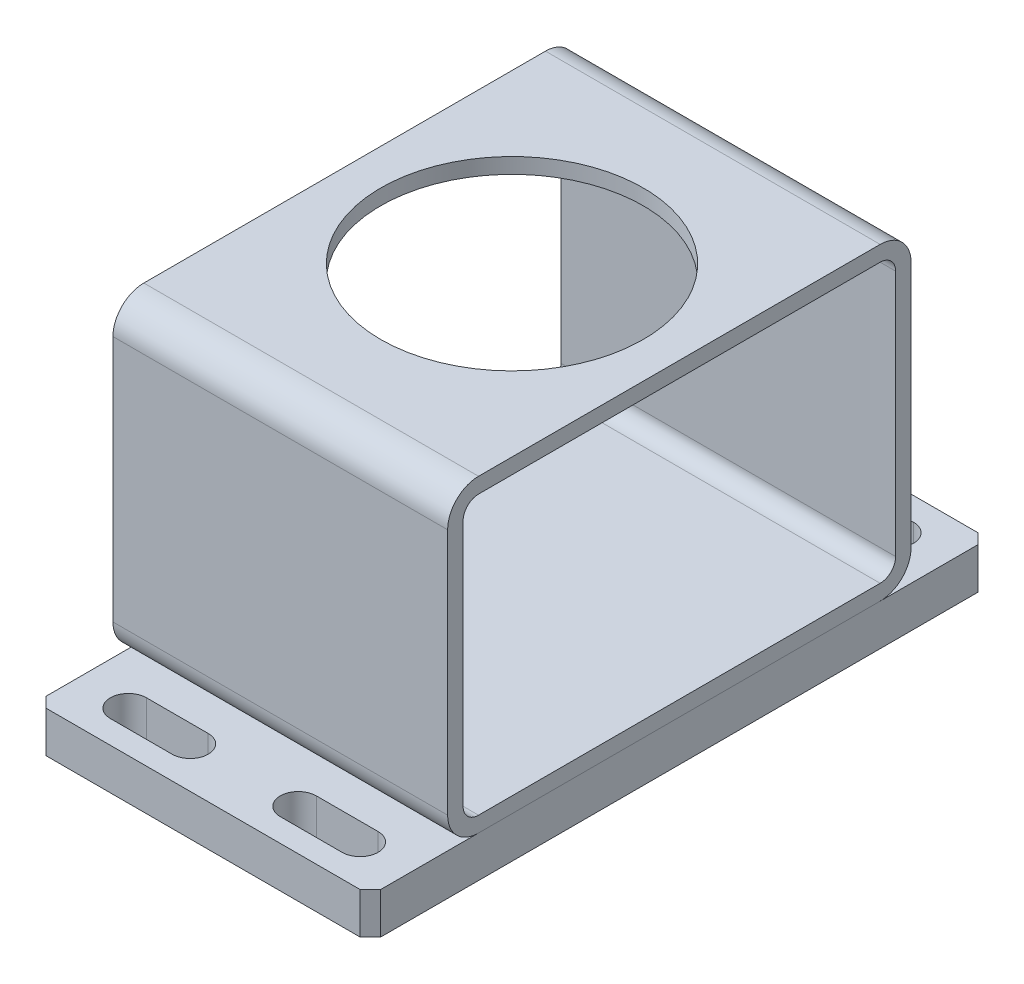
from build123d import *

# Parameters (mm, degrees)
GB_T6728_2002_90_X_60_X_3_1_DEPTH = 65
CUT_EXTRUDE_1_REACH               = 83.739
SKETCH_4_R                        = 25.5
SKETCH_7_W                        = 65
SKETCH_7_H                        = 120
EXTRUDE_1_DEPTH                   = 8
CUT_EXTRUDE_5_DEPTH               = 11
MIRROR_3_COPY_1_DEPTH             = 11
CHAMFER_1_SIZE                    = 2


with BuildPart() as part:
    # Sketch11 → 冷弯空心矩管gb∕t6728-2002 90 X 60 X 3(1) (new body)
    with BuildSketch(Plane.YZ.offset(-32.5)):
        with BuildLine():
            Line((-24, -45), (24, -45))
            ThreePointArc((24, -45), (28.242640687, -43.242640687), (30, -39))
            Line((30, -39), (30, 39))
            ThreePointArc((30, 39), (28.242640687, 43.242640687), (24, 45))
            Line((24, 45), (-24, 45))
            ThreePointArc((-24, 45), (-28.242640687, 43.242640687), (-30, 39))
            Line((-30, 39), (-30, -39))
            ThreePointArc((-30, -39), (-28.242640687, -43.242640687), (-24, -45))
        make_face()
        with BuildLine():
            Line((-24, -42), (24, -42))
            ThreePointArc((24, -42), (26.121320344, -41.121320344), (27, -39))
            Line((27, -39), (27, 39))
            ThreePointArc((27, 39), (26.121320344, 41.121320344), (24, 42))
            Line((24, 42), (-24, 42))
            ThreePointArc((-24, 42), (-26.121320344, 41.121320344), (-27, 39))
            Line((-27, 39), (-27, -39))
            ThreePointArc((-27, -39), (-26.121320344, -41.121320344), (-24, -42))
        make_face(mode=Mode.SUBTRACT)
    extrude(amount=GB_T6728_2002_90_X_60_X_3_1_DEPTH)

    # 草图4 → 切除-拉伸1 (cut, up to next)
    with BuildSketch(Plane(origin=(0, 30, 0), x_dir=(1, 0, 0), z_dir=(0, 1, 0)), mode=Mode.PRIVATE) as cut_extrude_1_sk1:
        with Locations(Location((0, 0, 0), (0, 0, 270))):
            Circle(SKETCH_4_R)
    cut_extrude_1_tool1 = extrude(cut_extrude_1_sk1.sketch, amount=-CUT_EXTRUDE_1_REACH, mode=Mode.PRIVATE) & part.part
    add(cut_extrude_1_tool1.solids().sort_by_distance((0, 30, 0))[0], mode=Mode.SUBTRACT)


with BuildPart() as body_2:
    # 草图7 → 凸台-拉伸1 (new body)
    with BuildSketch(Plane.XZ.offset(30)):
        Rectangle(SKETCH_7_W, SKETCH_7_H)
    extrude(amount=EXTRUDE_1_DEPTH)

    # 草图8 → 切除-拉伸5 (cut)
    with BuildSketch(Plane.XZ.offset(38)):
        with BuildLine():
            Line((-22.5, 55.5), (-10.5, 55.5))
            ThreePointArc((-10.5, 55.5), (-7, 52), (-10.5, 48.5))
            Line((-10.5, 48.5), (-22.5, 48.5))
            ThreePointArc((-22.5, 48.5), (-26, 52), (-22.5, 55.5))
        make_face()
    cut_extrude_5 = extrude(amount=-CUT_EXTRUDE_5_DEPTH, mode=Mode.SUBTRACT)

    # 镜向2: 切除-拉伸5 across plane
    add(cut_extrude_5.mirror(Plane(origin=(0, 0, 0), x_dir=(0, 0, 1), z_dir=(1, 0, 0))), mode=Mode.SUBTRACT)

    # 镜向3: 切除-拉伸5 across plane
    add(cut_extrude_5.mirror(Plane.XY), mode=Mode.SUBTRACT)

    # 镜向3 copy 1 sketch → 镜向3 copy 1 (cut)
    with BuildSketch(Plane(origin=(0, -38, 0), x_dir=(-1, 0, 0), z_dir=(0, -1, 0))):
        with BuildLine():
            Line((-22.5, 55.5), (-10.5, 55.5))
            ThreePointArc((-10.5, 55.5), (-7, 52), (-10.5, 48.5))
            Line((-10.5, 48.5), (-22.5, 48.5))
            ThreePointArc((-22.5, 48.5), (-26, 52), (-22.5, 55.5))
        make_face()
    extrude(amount=-MIRROR_3_COPY_1_DEPTH, mode=Mode.SUBTRACT)

    # 倒角1
    chamfer_1_edges = [body_2.edges().sort_by_distance(p)[0] for p in [
        (32.5, -34, -60),
        (-32.5, -34, -60),
        (-32.5, -34, 60),
        (32.5, -34, 60),
    ]]
    chamfer(chamfer_1_edges, length=CHAMFER_1_SIZE)


solid = Compound([part.part, body_2.part])
